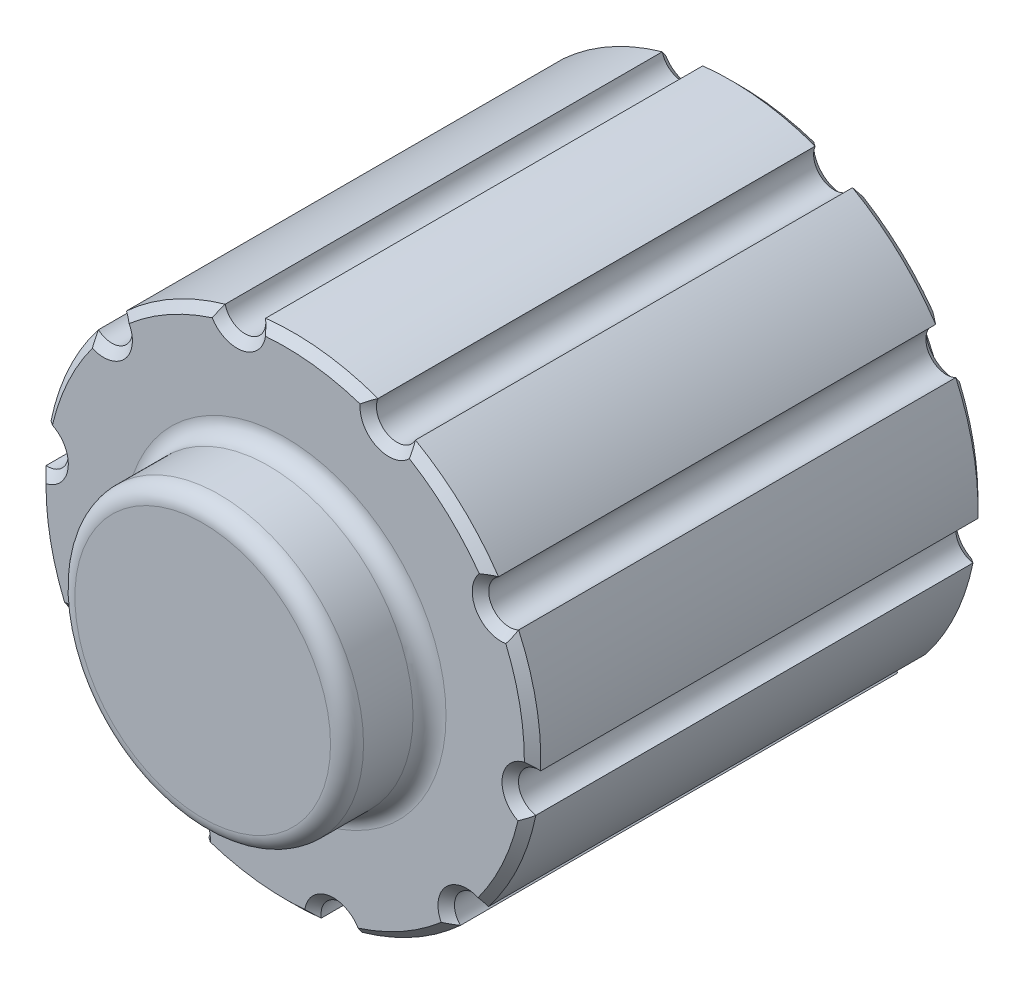
SolidWorks part; units mm, degrees
ref_plane "Front Plane" through (0, 0, 0) normal (0, 0, 1) x (1, 0, 0)
ref_plane "Top Plane" through (0, 0, 0) normal (0, 1, 0) x (1, 0, 0)
ref_plane "Right Plane" through (0, 0, 0) normal (1, 0, 0) x (0, 0, -1)
sketch "Sketch1" plane through (0, 0, 0) normal (0, 0, 1) x (1, 0, 0)
  circle A1 centre (-119, -40) radius 20
  circle A2 centre (-119, -40) radius 20
  dimension "D1" = 0
extrude "Boss-Extrude1" add sketch "Sketch1" along normal blind 5
sketch "Sketch2" plane through (0, 0, 5) normal (0, 0, 1) x (1, 0, 0)
  circle A2 centre (-119, -40) radius 30
  circle A3 centre (-119, -40) radius 30
  dimension "D1" = 10
extrude "Boss-Extrude2" add sketch "Sketch2" along normal blind 55
sketch "Sketch3" plane through (0, 0, 60) normal (0, 0, 1) x (1, 0, 0)
  circle A0 centre (-92.8215, -25.3478) radius 2.5
  circle A1 centre (-119, -40) radius 30 construction
  circle A11 centre (-89.2088, -43.5335) radius 2.5
  circle A12 centre (-96.9754, -60.3695) radius 2.5
  circle A13 centre (-113.1546, -69.425) radius 2.5
  circle A14 centre (-131.5665, -67.2412) radius 2.5
  circle A15 centre (-145.1785, -54.6522) radius 2.5
  circle A16 centre (-148.7912, -36.4665) radius 2.5
  circle A17 centre (-141.0246, -19.6305) radius 2.5
  circle A18 centre (-124.8454, -10.575) radius 2.5
  circle A19 centre (-106.4335, -12.7588) radius 2.5
  point P24 (-119, -40)
  dimension "D1" = 5
extrude "Cut-Extrude1" cut sketch "Sketch3" against normal blind 55
chamfer "Chamfer1" distance 1 angle 45 41 edges at (-98.6305, -17.9754, 5) (-89.575, -34.1546, 5) (-95.003, -26.5689, 5) (-99, -40, 5) (-89.575, -34.1546, 60) (-98.6305, -17.9754, 60) (-95.003, -26.5689, 60) (-139.1892, -21.328, 5) (-146.2412, -27.4335, 5) (-146.3086, -36.761, 5) (-148.425, -45.8454, 5) (-142.997, -53.4311, 5) (-139.3695, -62.0246, 5) (-130.5193, -64.9711, 5) (-122.5335, -69.7912, 5) (-113.6417, -66.9729, 5) (-104.3478, -66.1785, 5) (-98.8108, -58.672, 5) (-91.7588, -52.5665, 5) (-91.6914, -43.239, 5) (-107.4807, -15.0289, 5) (-115.4665, -10.2088, 5) (-124.3583, -13.0271, 5) (-133.6522, -13.8215, 5) (-115.4665, -10.2088, 60) (-107.4807, -15.0289, 60) (-91.6914, -43.239, 60) (-91.7588, -52.5665, 60) (-98.8108, -58.672, 60) (-104.3478, -66.1785, 60) (-113.6417, -66.9729, 60) (-122.5335, -69.7912, 60) (-130.5193, -64.9711, 60) (-139.3695, -62.0246, 60) (-142.997, -53.4311, 60) (-148.425, -45.8454, 60) (-146.3086, -36.761, 60) (-146.2412, -27.4335, 60) (-139.1892, -21.328, 60) (-133.6522, -13.8215, 60) (-124.3583, -13.0271, 60)
sketch "Sketch4" plane through (0, 0, 60) normal (0, 0, 1) x (1, 0, 0)
  circle A0 centre (-119, -40) radius 17.5
  dimension "D1" = 35
extrude "Boss-Extrude3" add sketch "Sketch4" along normal blind 10
fillet "Fillet1" radius 2 2 edges at (-101.5, -40, 70) (-101.5, -40, 60)
